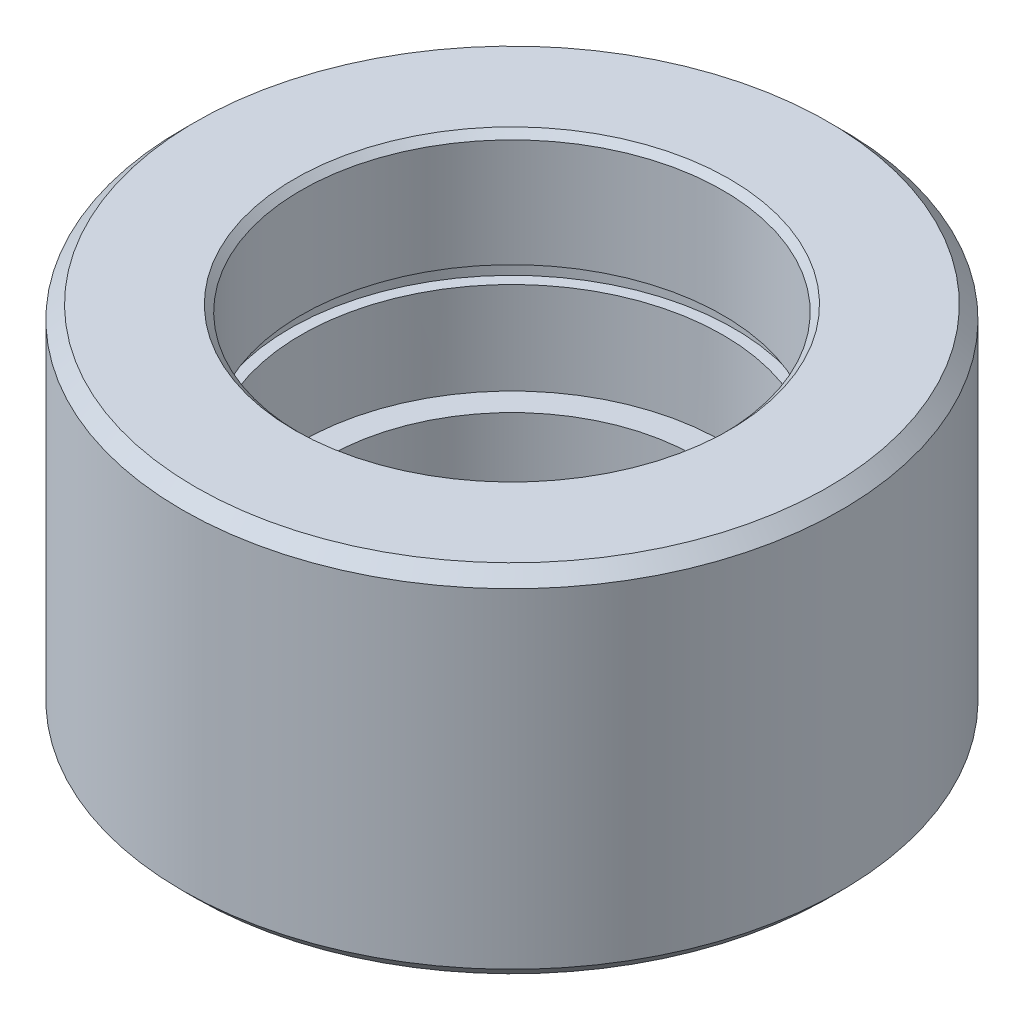
from build123d import *

# Parameters (mm, degrees)
SKETCH_1_R          = 25
EXTRUDE_1_DEPTH     = 27
SKETCH_2_R          = 16
CUT_EXTRUDE_1_DEPTH = 17
SKETCH_3_R          = 14
CUT_EXTRUDE_2_DEPTH = 40.230090492
CHAMFER_1_SIZE      = 1
CHAMFER_2_SIZE      = 0.5
SKETCH_4_W          = 2
SKETCH_4_H          = 1.3


with BuildPart() as part:
    # 草图1 → 凸台-拉伸1 (new body)
    with BuildSketch(Plane(origin=(0, 0, 0), x_dir=(1, 0, 0), z_dir=(0, 1, 0))):
        with Locations(Location((0, 0, 0), (0, 0, 270))):
            Circle(SKETCH_1_R)
    extrude(amount=EXTRUDE_1_DEPTH)

    # 草图2 → 切除-拉伸1 (cut)
    with BuildSketch(Plane(origin=(0, 27, 0), x_dir=(1, 0, 0), z_dir=(0, 1, 0))):
        with Locations(Location((0, 0, 0), (0, 0, 270))):
            Circle(SKETCH_2_R)
    extrude(amount=-CUT_EXTRUDE_1_DEPTH, mode=Mode.SUBTRACT)

    # 草图3 → 切除-拉伸2 (cut, through all)
    with BuildSketch(Plane(origin=(0, 10, 0), x_dir=(1, 0, 0), z_dir=(0, 1, 0))):
        with Locations(Location((0, 0, 0), (0, 0, 270))):
            Circle(SKETCH_3_R)
    extrude(amount=-CUT_EXTRUDE_2_DEPTH, mode=Mode.SUBTRACT)

    # 倒角1
    chamfer_1_edges = [part.edges().sort_by_distance(p)[0] for p in [
        (0, 0, -25),
        (0, 27, -25),
    ]]
    chamfer(chamfer_1_edges, length=CHAMFER_1_SIZE)

    # 倒角2
    chamfer_2_edges = [part.edges().sort_by_distance(p)[0] for p in [
        (0, 27, -16),
    ]]
    chamfer(chamfer_2_edges, length=CHAMFER_2_SIZE)

    # 草图4 → 切除-旋转1 (revolve, cut)
    with BuildSketch(Plane(origin=(0, 0, 0), x_dir=(0, 0, -1), z_dir=(1, 0, 0))):
        with Locations((-15.85, 17.65)):
            Rectangle(SKETCH_4_W, SKETCH_4_H)
    revolve(axis=Axis((0, 27, 0), (0, -1, 0)), mode=Mode.SUBTRACT)


solid = part.part
